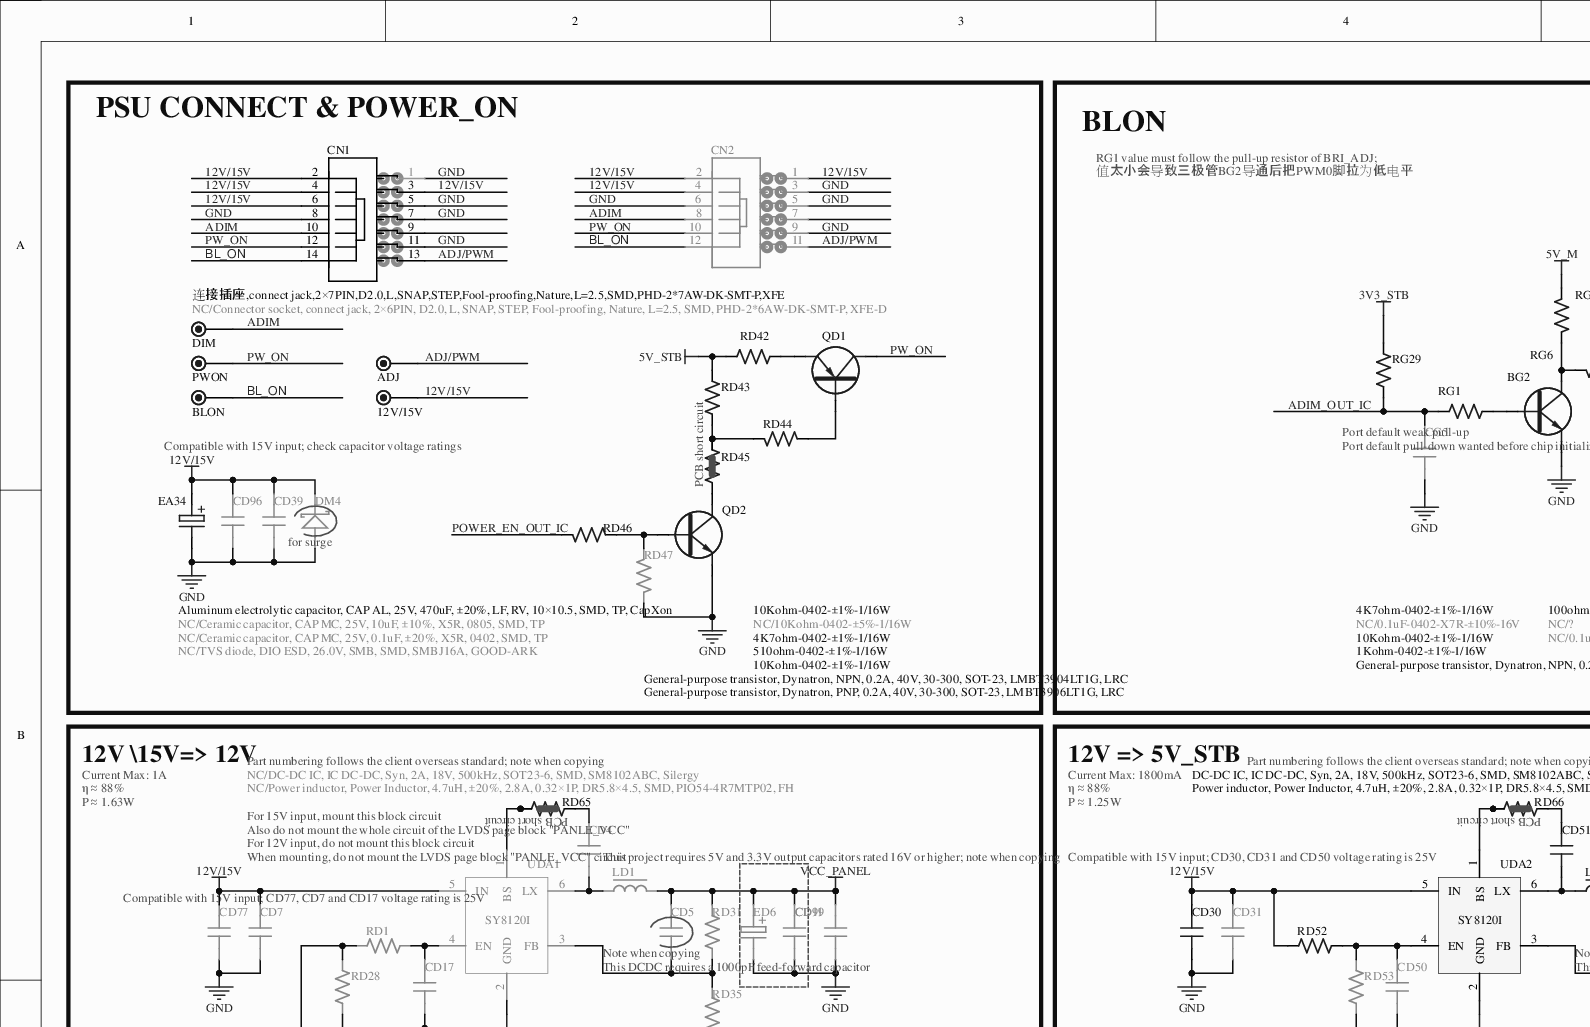
[diagram p0: MISC105950-35.SchDoc, top left]
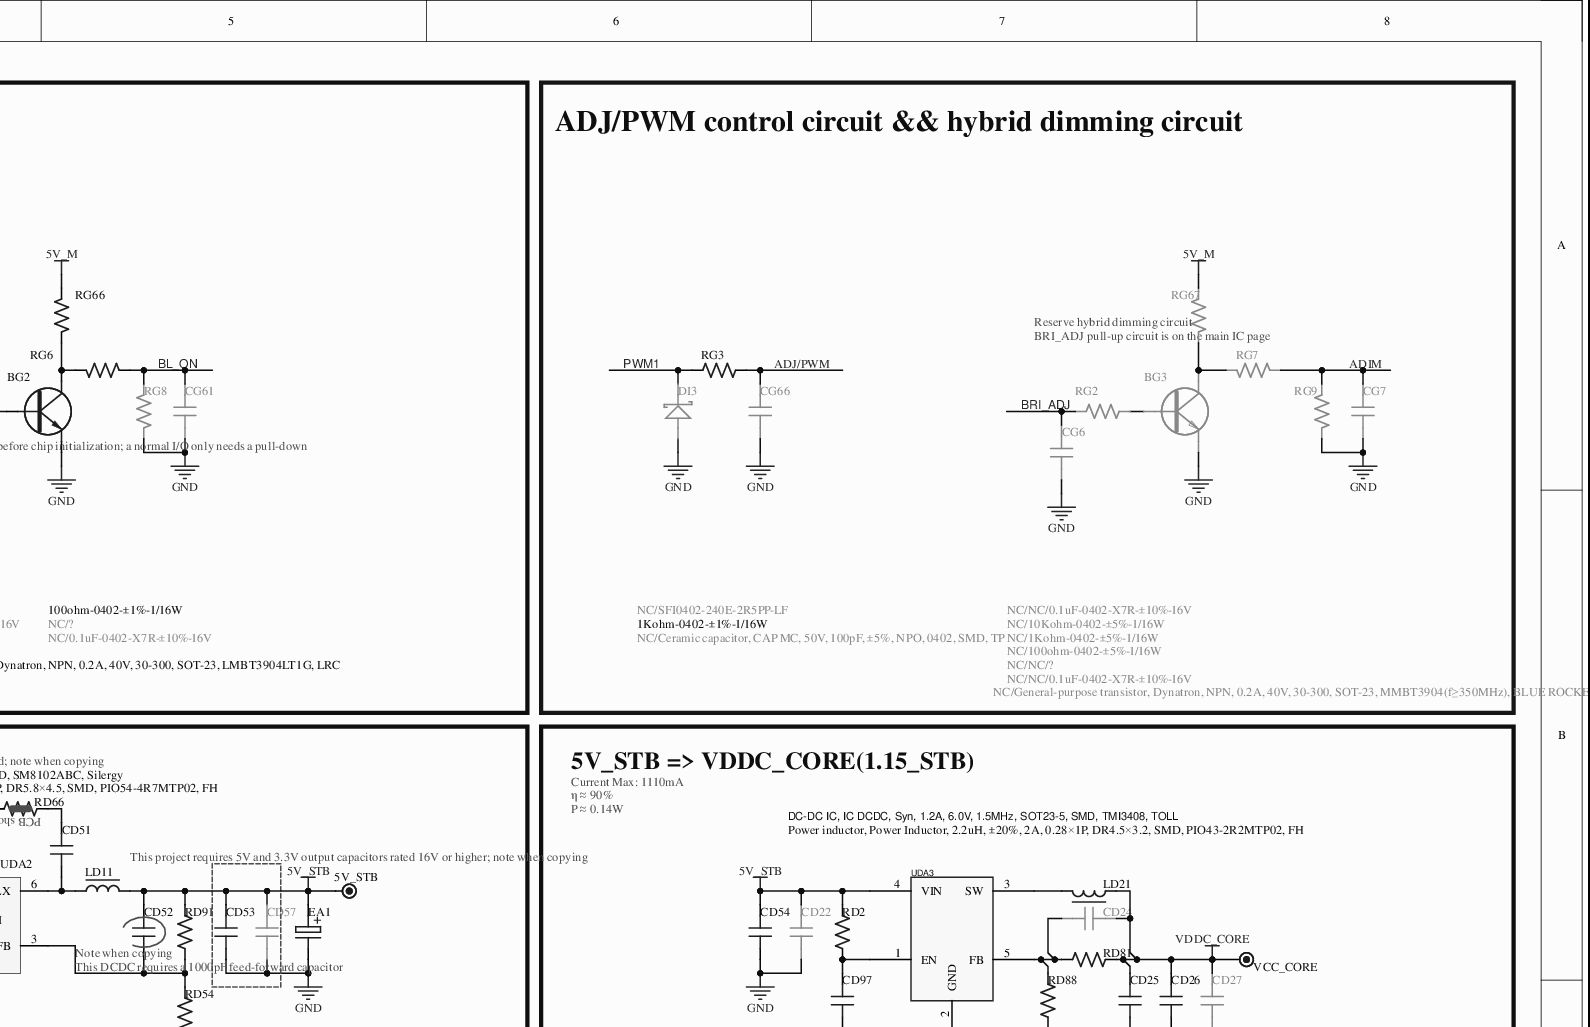
[diagram p1: MISC105950-35.SchDoc, top right]
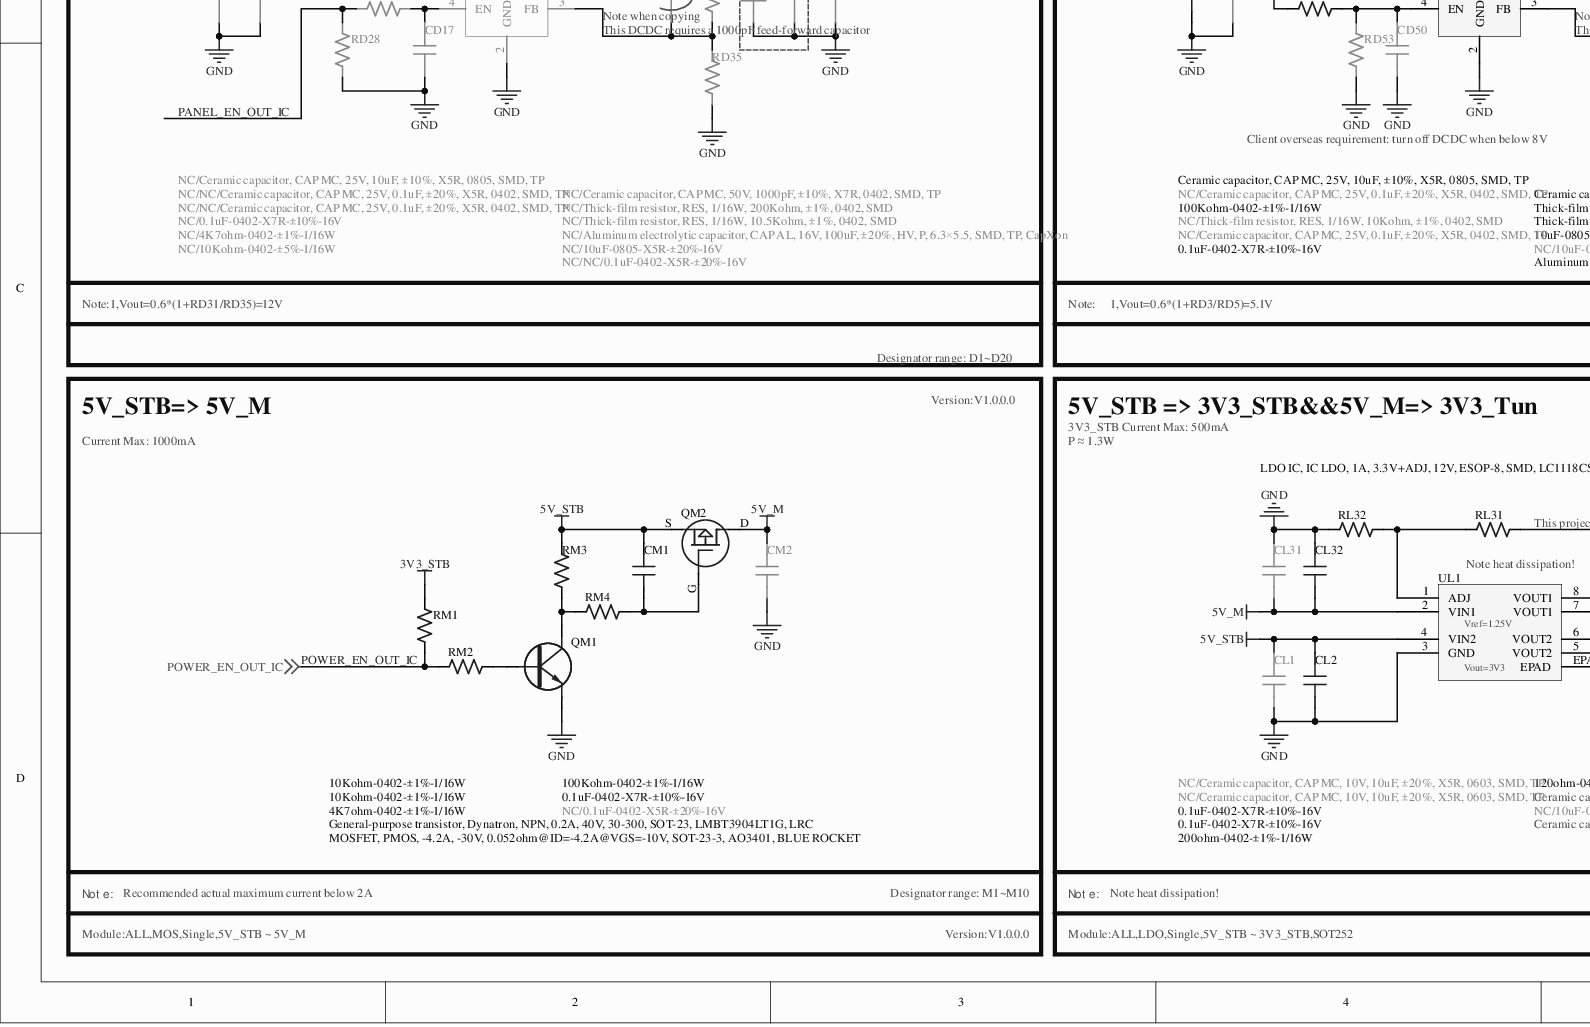
[diagram p2: MISC105950-35.SchDoc, bottom left]
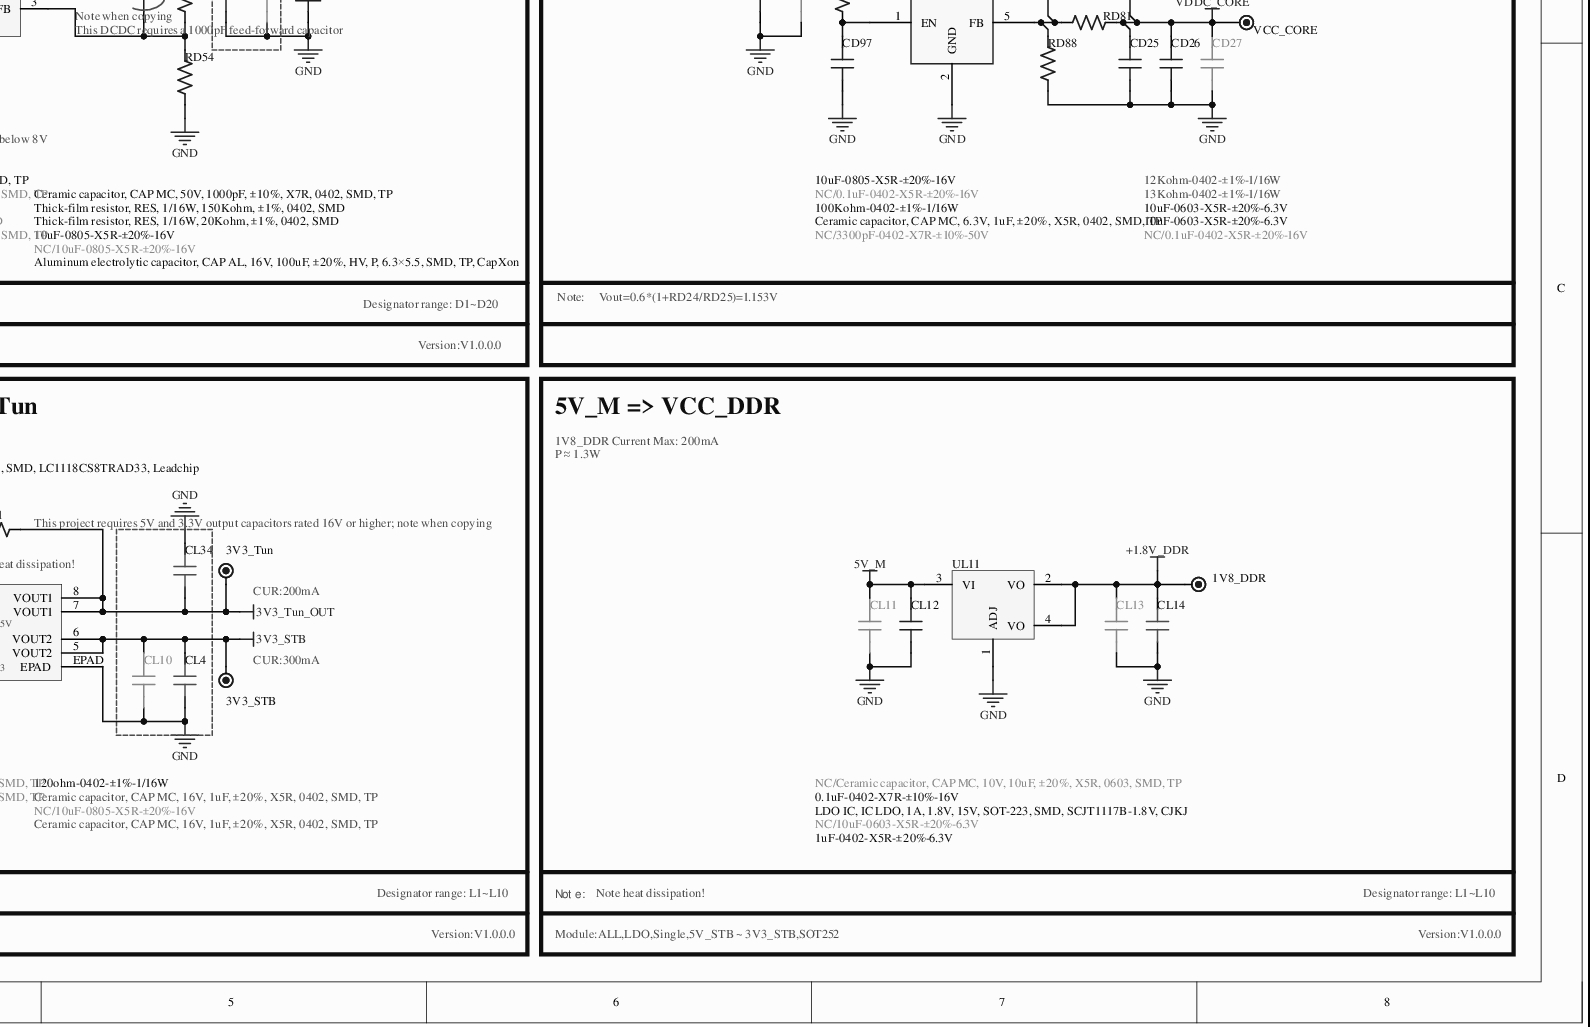
[diagram p3: MISC105950-35.SchDoc, bottom right]
# Altium project MISC105950-48.PrjPCB (part 3 of 8)

## Sheet MISC105950-35.SchDoc
size 571 x 363 mm

### Parts
1V8_DDR  TEST  [TP]  (value not drawn)
3V3_STB  TEST  [TP]  (value not drawn)
3V3_Tun  TEST  [TP]  (value not drawn)
5V_STB  TEST  [TP]  (value not drawn)
12V/15V  TEST  [TP]  (value not drawn)
ADJ  TEST  [TP]  (value not drawn)
BG2  General-purpose transistor, Dynatron, NPN, 0.2A, 40V, 30-300, SOT-23, LMBT3904LT1G, LRC  [SOT-23]
BG3  NC/General-purpose transistor, Dynatron, NPN, 0.2A, 40V, 30-300, SOT-23, MMBT3904(f≥350MHz), BLUE ROCKET  [SOT-23]
BLON  TEST  [TP]  (value not drawn)
CD4  NC/0.1uF-0402-X7R-±10%-16V  [C0402]
CD5  NC/Ceramic capacitor, CAP MC, 50V, 1000pF, ±10%, X7R, 0402, SMD, TP  [C0402]
CD7  NC/NC/Ceramic capacitor, CAP MC, 25V, 0.1uF, ±20%, X5R, 0402, SMD, TP  [C0402]
CD11  NC/NC/0.1uF-0402-X5R-±20%-16V  [C0402]
CD17  NC/NC/Ceramic capacitor, CAP MC, 25V, 0.1uF, ±20%, X5R, 0402, SMD, TP  [C0402]
CD22  NC/0.1uF-0402-X5R-±20%-16V  [C0402]
CD24  NC/3300pF-0402-X7R-±10%-50V  [C0402]
CD25  10uF-0603-X5R-±20%-6.3V  [C0603]
CD26  10uF-0603-X5R-±20%-6.3V  [C0603]
CD27  NC/0.1uF-0402-X5R-±20%-16V  [C0402]
CD30  Ceramic capacitor, CAP MC, 25V, 10uF, ±10%, X5R, 0805, SMD, TP  [C0805]
CD31  NC/Ceramic capacitor, CAP MC, 25V, 0.1uF, ±20%, X5R, 0402, SMD, TP  [C0402]
CD39  NC/Ceramic capacitor, CAP MC, 25V, 0.1uF, ±20%, X5R, 0402, SMD, TP  [C0402]
CD50  NC/Ceramic capacitor, CAP MC, 25V, 0.1uF, ±20%, X5R, 0402, SMD, TP  [C0402]
CD51  0.1uF-0402-X7R-±10%-16V  [C0402]
CD52  Ceramic capacitor, CAP MC, 50V, 1000pF, ±10%, X7R, 0402, SMD, TP  [C0402]
CD53  10uF-0805-X5R-±20%-16V  [C0805]
CD54  10uF-0805-X5R-±20%-16V  [C0805]
CD57  NC/10uF-0805-X5R-±20%-16V  [C0805]
CD77  NC/Ceramic capacitor, CAP MC, 25V, 10uF, ±10%, X5R, 0805, SMD, TP  [C0805]
CD96  NC/Ceramic capacitor, CAP MC, 25V, 10uF, ±10%, X5R, 0805, SMD, TP  [C0805]
CD97  Ceramic capacitor, CAP MC, 6.3V, 1uF, ±20%, X5R, 0402, SMD, TP  [C0402]
CD99  NC/10uF-0805-X5R-±20%-16V  [C0805]
CG5  NC/0.1uF-0402-X7R-±10%-16V  [C0402]
CG6  NC/NC/0.1uF-0402-X7R-±10%-16V  [C0402]
CG7  NC/NC/0.1uF-0402-X7R-±10%-16V  [C0402]
CG61  NC/0.1uF-0402-X7R-±10%-16V  [C0402]
CG66  NC/Ceramic capacitor, CAP MC, 50V, 100pF, ±5%, NPO, 0402, SMD, TP  [C0402]
CL1  NC/Ceramic capacitor, CAP MC, 10V, 10uF, ±20%, X5R, 0603, SMD, TP  [C0603]
CL2  0.1uF-0402-X7R-±10%-16V  [C0402]
CL4  Ceramic capacitor, CAP MC, 16V, 1uF, ±20%, X5R, 0402, SMD, TP  [C0402]
CL10  NC/10uF-0805-X5R-±20%-16V  [C0805]
CL11  NC/Ceramic capacitor, CAP MC, 10V, 10uF, ±20%, X5R, 0603, SMD, TP  [C0603]
CL12  0.1uF-0402-X7R-±10%-16V  [C0402]
CL13  NC/10uF-0603-X5R-±20%-6.3V  [C0603]
CL14  1uF-0402-X5R-±20%-6.3V  [C0402]
CL31  NC/Ceramic capacitor, CAP MC, 10V, 10uF, ±20%, X5R, 0603, SMD, TP  [C0603]
CL32  0.1uF-0402-X7R-±10%-16V  [C0402]
CL34  Ceramic capacitor, CAP MC, 16V, 1uF, ±20%, X5R, 0402, SMD, TP  [C0402]
CM1  0.1uF-0402-X7R-±10%-16V  [C0402]
CM2  NC/0.1uF-0402-X5R-±20%-16V  [C0402]
CN1  连接插座,connect jack,2×7PIN,D2.0,L,SNAP,STEP,Fool-proofing,Nature,L=2.5,SMD,PHD-2*7AW-DK-SMT-P,XFE  [SIP2*7H/2.0D-LS]
CN2  NC/Connector socket, connect jack, 2×6PIN, D2.0, L, SNAP, STEP, Fool-proofing, Nature, L=2.5, SMD, PHD-2*6AW-DK-SMT-P, XFE-D  [SIP2*6H/2.0D-LS]
DI3  NC/SFI0402-240E-2R5PP-LF  [DIODE-S0402]
DIM  TEST  [TP]  (value not drawn)
DM4  NC/TVS diode, DIO ESD, 26.0V, SMB, SMD, SMBJ16A, GOOD-ARK  [DIODE-SMB-2]
EA1  Aluminum electrolytic capacitor, CAP AL, 16V, 100uF, ±20%, HV, P, 6.3×5.5, SMD, TP, CapXon  [EC(6.5*5.5)-S]
EA34  Aluminum electrolytic capacitor, CAP AL, 25V, 470uF, ±20%, LF, RV, 10×10.5, SMD, TP, CapXon  [EC(10*10.5)-S]
ED6  NC/Aluminum electrolytic capacitor, CAP AL, 16V, 100uF, ±20%, HV, P, 6.3×5.5, SMD, TP, CapXon  [EC(6.5*5.5)-S]
LD1  NC/Power inductor, Power Inductor, 4.7uH, ±20%, 2.8A, 0.32×1P, DR5.8×4.5, SMD, PIO54-4R7MTP02, FH  [L(5.8*4.5)-S]
LD11  Power inductor, Power Inductor, 4.7uH, ±20%, 2.8A, 0.32×1P, DR5.8×4.5, SMD, PIO54-4R7MTP02, FH  [L(5.8*4.5)-S]
LD21  Power inductor, Power Inductor, 2.2uH, ±20%, 2A, 0.28×1P, DR4.5×3.2, SMD, PIO43-2R2MTP02, FH  [L(4.5*3.5)-S]
PWON  TEST  [TP]  (value not drawn)
QD1  General-purpose transistor, Dynatron, PNP, 0.2A, 40V, 30-300, SOT-23, LMBT3906LT1G, LRC  [SOT-23]
QD2  General-purpose transistor, Dynatron, NPN, 0.2A, 40V, 30-300, SOT-23, LMBT3904LT1G, LRC  [SOT-23]
QM1  General-purpose transistor, Dynatron, NPN, 0.2A, 40V, 30-300, SOT-23, LMBT3904LT1G, LRC  [SOT-23]
QM2  MOSFET, PMOS, -4.2A, -30V, 0.052ohm@ID=-4.2A@VGS=-10V, SOT-23-3, AO3401, BLUE ROCKET  [SOT-23-1]
RD1  NC/10Kohm-0402-±5%-1/16W  [R0402]
RD2  100Kohm-0402-±1%-1/16W  [R0402]
RD28  NC/4K7ohm-0402-±1%-1/16W  [R0402]
RD31  NC/Thick-film resistor, RES, 1/16W, 200Kohm, ±1%, 0402, SMD  [R0402]
RD35  NC/Thick-film resistor, RES, 1/16W, 10.5Kohm, ±1%, 0402, SMD  [R0402]
RD42  510ohm-0402-±1%-1/16W  [R0402]
RD43  4K7ohm-0402-±1%-1/16W  [R0402]
RD44  10Kohm-0402-±1%-1/16W  [R0402]
RD45  NC/0ohm-0402-PCB  [R0402SC]  (value not drawn)
RD46  10Kohm-0402-±1%-1/16W  [R0402]
RD47  NC/10Kohm-0402-±5%-1/16W  [R0402]
RD52  100Kohm-0402-±1%-1/16W  [R0402]
RD53  NC/Thick-film resistor, RES, 1/16W, 10Kohm, ±1%, 0402, SMD  [R0402]
RD54  Thick-film resistor, RES, 1/16W, 20Kohm, ±1%, 0402, SMD  [R0402]
RD65  NC/0ohm-0402-PCB  [R0402SC]  (value not drawn)
RD66  NC/0ohm-0402-PCB  [R0402SC]  (value not drawn)
RD81  12Kohm-0402-±1%-1/16W  [R0402]
RD88  13Kohm-0402-±1%-1/16W  [R0402]
RD91  Thick-film resistor, RES, 1/16W, 150Kohm, ±1%, 0402, SMD  [R0402]
RG1  10Kohm-0402-±1%-1/16W  [R0402]
RG2  NC/10Kohm-0402-±5%-1/16W  [R0402]
RG3  1Kohm-0402-±1%-1/16W  [R0402]
RG6  100ohm-0402-±1%-1/16W  [R0402]
RG7  NC/100ohm-0402-±5%-1/16W  [R0402]
RG8  NC/?  [R0402]
RG9  NC/NC/?  [R0402]
RG29  4K7ohm-0402-±1%-1/16W  [R0402]
RG66  1Kohm-0402-±1%-1/16W  [R0402]
RG67  NC/1Kohm-0402-±5%-1/16W  [R0402]
RL31  120ohm-0402-±1%-1/16W  [R0402]
RL32  200ohm-0402-±1%-1/16W  [R0402]
RM1  10Kohm-0402-±1%-1/16W  [R0402]
RM2  10Kohm-0402-±1%-1/16W  [R0402]
RM3  4K7ohm-0402-±1%-1/16W  [R0402]
RM4  100Kohm-0402-±1%-1/16W  [R0402]
UDA1  NC/DC-DC IC, IC DC-DC, Syn, 2A, 18V, 500kHz, SOT23-6, SMD, SM8102ABC, Silergy  [SOT23-6-2]
UDA2  DC-DC IC, IC DC-DC, Syn, 2A, 18V, 500kHz, SOT23-6, SMD, SM8102ABC, Silergy  [SOT23-6-2]
UDA3  DC-DC IC, IC DCDC, Syn, 1.2A, 6.0V, 1.5MHz, SOT23-5, SMD, TMI3408, TOLL  [SOT-23-5]
UL1  LDO IC, IC LDO, 1A, 3.3V+ADJ, 12V, ESOP-8, SMD, LC1118CS8TRAD33, Leadchip  [SOP8/1.27-3]
UL11  LDO IC, IC LDO, 1A, 1.8V, 15V, SOT-223, SMD, SCJT1117B-1.8V, CJKJ  [SOT-223]
VCC_CORE  TEST  [TP]  (value not drawn)

### Blocks framed on the sheet
PSU CONNECT & POWER_ON: 12V/15V ADJ BLON CD39 CD96 CN1 CN2 DIM DM4 EA34 PWON QD1 QD2 RD42-RD47
BLON: BG2 CG5 CG61 RG1 RG6 RG8 RG29 RG66
ADJ/PWM control circuit && hybrid dimming circuit: BG3 CG6 CG7 CG66 DI3 RG2 RG3 RG7 RG9 RG67
5V_STB => VDDC_CORE(1.15_STB): CD22 CD24-CD27 CD54 CD97 LD21 RD2 RD81 RD88 UDA3 VCC_CORE
12V \15V=> 12V: CD4 CD5 CD7 CD11 CD17 CD77 CD99 ED6 LD1 RD1 RD28 RD31 RD35 RD65 UDA1
12V => 5V_STB: 5V_STB CD30 CD31 CD50-CD53 CD57 EA1 LD11 RD52-RD54 RD66 RD91 UDA2
5V_STB=> 5V_M: CM1 CM2 QM1 QM2 RM1-RM4
5V_STB => 3V3_STB&&5V_M=> 3V3_Tun: 3V3_STB 3V3_Tun CL1 CL2 CL4 CL10 CL31 CL32 CL34 RL31 RL32 UL1
5V_M => VCC_DDR: 1V8_DDR CL11-CL14 UL11

### Nets
3V3_STB: 3V3_STB.1 CL4.1 CL10.1 RG29.2 RM1.2 UL1.5(VOUT2) UL1.6(VOUT2)
3V3_Tun_OUT: 3V3_Tun.1 CL34.2 RL31.2 UL1.7(VOUT1) UL1.8(VOUT1)
5V_M: CL11.2 CL12.2 CL31.1 CL32.1 CM2.2 QM2.D RG66.2 RG67.2 UL1.2(VIN1) UL11.3(VI)
5V_STB: 5V_STB.1 CD22.2 CD52.2 CD53.1 CD54.1 CD57.1 CL1.2 CL2.2 CM1.2 EA1.1 LD11.2 QM2.S RD2.1 RD42.2 RD43.2 RD91.2 RM3.2 UDA3.4(VIN) UL1.4(VIN2)
12V/15V: 12V/15V.1 CD7.1 CD30.2 CD31.1 CD39.1 CD77.2 CD96.2 CN1.2 CN1.3 CN1.4 CN1.6 CN2.1 CN2.2 CN2.4 DM4.K EA34.1 RD52.1 UDA1.5(IN) UDA2.5(IN)
+1.8V_DDR: 1V8_DDR.1 CL13.2 CL14.2 UL11.2(VO) UL11.4(VO)
GND: BG2.E BG3.E CD7.2 CD11.1 CD17.2 CD22.1 CD25.1 CD26.1 CD27.1 CD30.1 CD31.2 CD39.2 CD50.2 CD53.2 CD54.2 CD57.2 CD77.1 CD96.1 CD97.2 CD99.2 CG5.1 CG6.1 CG7.1 CG61.1 CG66.1 CL1.1 CL2.1 CL4.2 CL10.2 CL11.1 CL12.1 CL13.1 CL14.1 CL31.2 CL32.2 CL34.1 CM2.1 CN1.1 CN1.5 CN1.7 CN1.8 CN1.11 CN2.3 CN2.5 CN2.6 CN2.9 DI3.A DM4.A EA1.2 EA34.2 ED6.2 QD2.E QM1.E RD28.1 RD35.1 RD47.2 RD53.2 RD54.1 RD88.1 RG8.1 RG9.1 RL32.1 UDA1.2(GND) UDA2.2(GND) UDA3.2(GND) UL1.3(GND) UL1.EPAD UL11.1(ADJ)
VCC_PANEL: CD5.2 CD11.2 CD99.1 ED6.1 LD1.2 RD31.2
VDDC_CORE: CD24.2 CD25.2 CD26.2 CD27.2 LD21.1 RD81.2 VCC_CORE.1
ADIM: CG7.2 CN1.10 CN2.8 DIM.1 RG7.1 RG9.2
ADIM_OUT_IC: CG5.2 RG1.2 RG29.1
ADJ/PWM: ADJ.1 CG66.2 CN1.13 CN2.11 RG3.1
BL_ON: BLON.1 CG61.2 CN1.14 CN2.12 RG6.1 RG8.2
BRI_ADJ: CG6.2 RG2.2
PANEL_EN_OUT_IC: RD1.1 RD28.2
POWER_EN_OUT_IC: RD46.1 RM1.1 RM2.1 ; off-sheet POWER_EN_OUT_IC
PW_ON: CN1.12 CN2.10 PWON.1 QD1.C
PWM1: DI3.K RG3.2
NetBG2_B: BG2.B RG1.1
NetBG2_C: BG2.C RG6.2 RG66.1
NetBG3_B: BG3.B RG2.1
NetBG3_C: BG3.C RG7.2 RG67.1
NetCD4_1: CD4.1 LD1.1 UDA1.6(LX)
NetCD4_2: CD4.2 RD65.1
NetCD5_1: CD5.1 RD31.1 RD35.2 UDA1.3(FB)
NetCD17_1: CD17.1 RD1.2 UDA1.4(EN)
NetCD24_1: CD24.1 RD81.1 RD88.2 UDA3.5(FB)
NetCD50_1: CD50.1 RD52.2 RD53.1 UDA2.4(EN)
NetCD51_1: CD51.1 LD11.1 UDA2.6(LX)
NetCD51_2: CD51.2 RD66.1
NetCD52_1: CD52.1 RD54.2 RD91.1 UDA2.3(FB)
NetCD97_1: CD97.1 RD2.2 UDA3.1(EN)
NetCM1_1: CM1.1 QM2.G RM4.2
NetLD21_2: LD21.2 UDA3.3(SW)
NetQD1_B: QD1.B RD44.1
NetQD1_E: QD1.E RD42.1
NetQD2_B: QD2.B RD46.2 RD47.1
NetQD2_C: QD2.C RD45.1
NetQM1_B: QM1.B RM2.2
NetQM1_C: QM1.C RM3.1 RM4.1
NetRD43_1: RD43.1 RD44.2 RD45.2 RD45.3
NetRD65_2: RD65.2 RD65.3 UDA1.1(BS)
NetRD66_2: RD66.2 RD66.3 UDA2.1(BS)
NetRL31_1: RL31.1 RL32.2 UL1.1(ADJ)

Not connected (* = marked no-connect by the designer): CN1 9*; CN2 7*

### Notes on the sheet
- RG1 value must follow the pull-up resistor of BRI_ADJ;
- 值太小会导致三极管BG2导通后把PWM0脚拉为低电平
- (near RG67) BRI_ADJ pull-up circuit is on the main IC page
- (near RG67) Reserve hybrid dimming circuit
- Compatible with 15V input; check capacitor voltage ratings
- (near CG5) Port default weak pull-up
- Port default pull-down wanted before chip initialization; a normal I/O only needs a pull-down
- (near DM4) for surge
- η ≈ 88%
- P ≈ 1.63W
- Current Max: 1A
- Part numbering follows the client overseas standard; note when copying
- For 15V input, mount this block circuit
- P ≈ 1.25W
- Current Max: 1800mA
- η ≈ 90%
- P ≈ 0.14W
- Current Max: 1110mA
- (near CD4) Also do not mount the whole circuit of the LVDS page block "PANLE_VCC"
- For 12V input, do not mount this block circuit
- (near CD4) When mounting, do not mount the LVDS page block "PANLE_VCC" circuit
- (near CD4) This project requires 5V and 3.3V output capacitors rated 16V or higher; note when copying
- (near UDA2) Compatible with 15V input; CD30, CD31 and CD50 voltage rating is 25V
- This project requires 5V and 3.3V output capacitors rated 16V or higher; note when copying
- (near UDA1) Compatible with 15V input; CD77, CD7 and CD17 voltage rating is 25V
- (near CD5) Note when copying
- (near CD52) Note when copying
- This DCDC requires a 1000pF feed-forward capacitor
- Client overseas requirement: turn off DCDC when below 8V
- Note:
- Vout=0.6*(1+RD24/RD25)=1.153V
- 1,Vout=0.6*(1+RD31/RD35)=12V
- Designator range: D1~D20
- 1,Vout=0.6*(1+RD3/RD5)=5.1V
- Version:V1.0.0.0
- 3V3_STB Current Max: 500mA
- Current Max: 1000mA
- P ≈ 1.3W
- 1V8_DDR Current Max: 200mA
- Note heat dissipation!
- (near 3V3_Tun) CUR:200mA
- (near 3V3_STB) CUR:300mA
- Recommended actual maximum current below 2A
- Designator range: M1~M10
- Designator range: L1~L10
- Module:ALL,MOS,Single,5V_STB ~ 5V_M
- Module:ALL,LDO,Single,5V_STB ~ 3V3_STB,SOT252

### Library data of the parts
BG2 BG3 QD2 = LMBT3904LT1G-D-NPN: Q-NPN-#-#-#
CD4 CD51 CL2 CL12 CL32 CM1 CM2 = 004.003.0000403-D: Ceramic capacitor, CAP MC, 16V, 0.1uF, ±20%, X5R, 0402, SMD, TP-D
CD5 CD52 = 004.003.0000558-D: Ceramic capacitor, CAP MC, 50V, 470pF, ±5%, NPO, 0402, SMD, TP-D
CD7 CD17 CD31 CD39 CD50 = 004.003.0000814-D: Ceramic capacitor, CAP MC, 25V, 0.1uF, ±20%, X5R, 0402, SMD, TP-D
CD11 CD97 = 0.1uF-0402-Y5V-+80%-20%-16V-D
CD22 CD27 CG5-CG7 CG61 = 0.1uF-0402-X5R-±20%-16V-D
CD24 = 3300pF-0402-X7R-±10%-50V-D
CD25 CD26 = 10uF-0603-X5R-±20%-6.3V-D
CD30 CD77 CD96 = 10uF-0805-X5R-+15%-16V-D
CD53 CD54 CD57 CL10 = 004.003.0000386-D: Ceramic capacitor, CAP MC, 16V, 10uF, ±20%, X5R, 0805, SMD, TP-D
CD99 = 10uF-0805-X5R-±20%-16V-D
CG66 CL4 CL34 = 1uF-0402-X5R-±20%-6.3V-D
CL1 CL11 CL31 = 004.003.0000394-D: Ceramic capacitor, CAP MC, 10V, 10uF, ±20%, X5R, 0603, SMD, TP-D
CL13 = 004.003.0000383-D: Ceramic capacitor, CAP MC, 6.3V, 10uF, ±20%, X5R, 0603, SMD, TP-D
CL14 = 004.003.0000382-D: Ceramic capacitor, CAP MC, 6.3V, 1uF, ±20%, X5R, 0402, SMD, TP-D
CN1 = XXX.XXX.0003725: Connector socket, connect jack, 2×7PIN, D2.0, L, SNAP, STEP, Fool-proofing, Nature, L=2.5, SMD, PHD-2*7AW-DK-SMT-P, XFE-D
CN2 = XXX.XXX.0003724: Connector socket, connect jack, 2×6PIN, D2.0, L, SNAP, STEP, Fool-proofing, Nature, L=2.5, SMD, PHD-2*6AW-DK-SMT-P, XFE-D
DI3 = 004.005.0000315-D: TVS diode, DIO ESD, 2.5pF, 200V, 0402, SMD, SFI0402-240E-2R5PP-LF, SFI-D
DM4 = 004.005.0000611: TVS diode, DIO ESD, 19.9V, SMB, SMD, SMBFJ12A, LRC-D
EA1 ED6 = 004.003.0000405-D: Aluminum electrolytic capacitor, CAP AL, 16V, 100uF, ±20%, HV, P, 6.3×5.5, SMD, TP, CapXon-D
EA34 = 铝电解电容,CAP AL,100V,33uF,±20%,LF,RV,10×10.5,SMD,TP,CapXon-D: Electrolytic
LD1 LD11 = 004.004.0000017-D: Power inductor, Power Inductor, 4.7uH, ±20%, 2.8A, 0.35×1P, DR5.8×4.5, SMD, SCD54TL-4R7M, Soldier-D
LD21 = SLN43T-6R8M-D
QD1 = LMBT3906LT1G-D-PNP
QM1 = 004.006.0000007-D: General-purpose transistor, Dynatron, NPN, 0.2A, 40V, 60-300, SOT-23, KMBT3904, KEXIN-D
QM2 = 004.007.0000286-D: MOSFET, PMOS, -4.7A, -20V, 70mohm@ID=-4.7A@VGS=-4.5V, SOT23-LC, LPB3443LT1G, LRC-D
RD1 RD28 RD52 RD53 RM4 = 004.002.0000579-D: Thick-film resistor, RES, 1/16W, 100Kohm, ±5%, 0402, SMD-D
RD2 RD44 RD46 RD47 = 10Kohm-0402-±5%-1/16W-D
RD31 RD91 = 004.002.0000104-D: Thick-film resistor, RES, 1/16W, 33Kohm, ±1%, 0402, SMD-D
RD35 RD54 = 004.002.0000717-D: Thick-film resistor, RES, 1/16W, 6.04Kohm, ±1%, 0402, SMD-D
RD42 RG1 RG2 = 510ohm-0402-±5%-1/16W-D
RD43 = 1K5ohm-0402-±1%-1/16W-D
RD45 RD65 RD66 = 0ohm-0402-PCB-D
RD81 = 10Kohm-0402-±1%-1/16W-D
RD88 = 12Kohm-0402-±1%-1/16W-D
RG3 RG29 = 4K7ohm-0402-±5%-1/16W-D
RG6 RG7 = 33ohm-0402-±5%-1/16W-D
RG8 RG9 RG66 RG67 = 1Kohm-0402-±5%-1/16W-D
RL31 = 004.002.0000584-D: Thick-film resistor, RES, 1/16W, 120ohm, ±1%, 0402, SMD-D
RL32 = 004.002.0000616-D: Thick-film resistor, RES, 1/16W, 200ohm, ±1%, 0402, SMD-D
RM1 RM2 = 004.002.0000577-D: Thick-film resistor, RES, 1/16W, 10Kohm, ±5%, 0402, SMD-D
RM3 = 004.002.0000689-D: Thick-film resistor, RES, 1/16W, 4.7Kohm, ±5%, 0402, SMD-D
UDA1 UDA2 = 004.010.0001028-D: DC-DC IC, IC DC-DC, Syn, 2A, 18V, 500kHz, SOT23-6, SMD, SY8120IABC, Silergy-D
UDA3 = DC-DC芯片,IC DCDC,Syn,1.2A,7.0V,1.5MHz,SOT23-5,SMD,LC2127CB5TR,Leadchip-D
UL1 = 004.010.0000467-D: LDO IC, IC LDO, 1A, 3.3V+ADJ, 12V, ESOP-8, SMD, LC1118CS8TRAD33, Leadchip-D
UL11 = 004.010.0000061-D: LDO IC, IC LDO, 1A, 1.8V, 12V, SOT-223, SMD, LC1117CLTR18, Leadchip-D